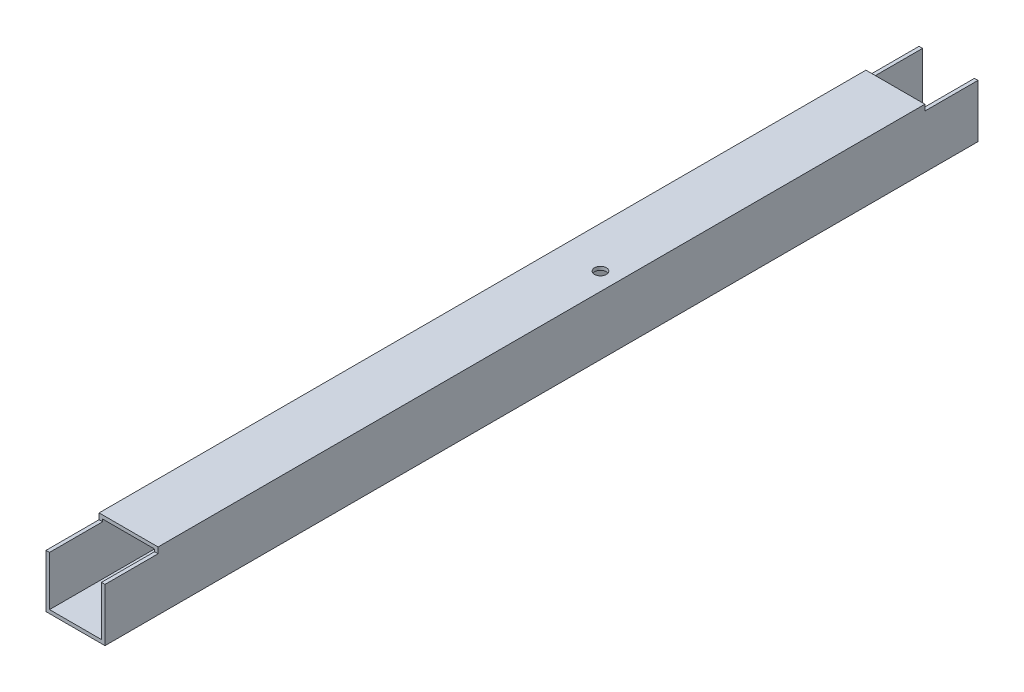
from build123d import *

# Parameters (mm, degrees)
SKETCH_1_W          = 50
SKETCH_1_H          = 50
SKETCH_1_W_2        = 44
SKETCH_1_H_2        = 44
EXTRUDE_1_DEPTH     = 790
SKETCH_2_W          = 50
SKETCH_2_H          = 45
CUT_EXTRUDE_1_DEPTH = 5
SKETCH_3_R          = 5
CUT_EXTRUDE_2_DEPTH = 5
CUT_EXTRUDE_3_DEPTH = 50
CUT_EXTRUDE_4_DEPTH = 50
EXTRUDE_2_DEPTH     = 25
EXTRUDE_3_DEPTH     = 25
CUT_EXTRUDE_5_DEPTH = 25
CUT_EXTRUDE_6_DEPTH = 25
SKETCH_10_R         = 5
CUT_EXTRUDE_7_DEPTH = 94


with BuildPart() as part:
    # 草图1 → 凸台-拉伸1 (new body)
    with BuildSketch(Plane.XY):
        with Locations((25, 25)):
            Rectangle(SKETCH_1_W, SKETCH_1_H)
        with Locations((25, 25)):
            Rectangle(SKETCH_1_W_2, SKETCH_1_H_2, mode=Mode.SUBTRACT)
    extrude(amount=EXTRUDE_1_DEPTH)

    # 草图2 → 切除-拉伸1 (cut)
    with BuildSketch(Plane(origin=(0, 50, 0), x_dir=(1, 0, 0), z_dir=(0, 1, 0))):
        with Locations((25, -22.5)):
            Rectangle(SKETCH_2_W, SKETCH_2_H)
        with Locations((25, -767.5)):
            Rectangle(SKETCH_2_W, SKETCH_2_H)
    extrude(amount=-CUT_EXTRUDE_1_DEPTH, mode=Mode.SUBTRACT)

    # 草图3 → 切除-拉伸2 (cut)
    with BuildSketch(Plane(origin=(0, 50, 0), x_dir=(1, 0, 0), z_dir=(0, 1, 0))):
        with Locations(Location((35, -330, 0), (0, 0, 270))):
            Circle(SKETCH_3_R)
    extrude(amount=-CUT_EXTRUDE_2_DEPTH, mode=Mode.SUBTRACT)

    # 草图4 → 切除-拉伸3 (cut)
    with BuildSketch(Plane.XY.offset(790)):
        Polygon((50, 0), (50, 45), (47, 45), (47, 3), (3, 3), (3, 45), (0, 45), (0, 0), align=None)
    extrude(amount=-CUT_EXTRUDE_3_DEPTH, mode=Mode.SUBTRACT)

    # 草图5 → 切除-拉伸4 (cut)
    with BuildSketch(Plane.XY.offset(745)):
        Polygon((47, 47), (47, 45), (50, 45), (50, 50), (0, 50), (0, 45), (3, 45), (3, 47), align=None)
    extrude(amount=-CUT_EXTRUDE_4_DEPTH, mode=Mode.SUBTRACT)

    # 草图6 → 凸台-拉伸2 (add)
    with BuildSketch(Plane.XY.offset(695)):
        Polygon((3, 47), (47, 47), (47, 45), (50, 45), (50, 50), (0, 50), (0, 45), (3, 45), align=None)
    extrude(amount=EXTRUDE_2_DEPTH)

    # 草图7 → 凸台-拉伸3 (add)
    with BuildSketch(Plane.XY.offset(740)):
        Polygon((0, 0), (50, 0), (50, 45), (47, 45), (47, 3), (3, 3), (3, 45), (0, 45), align=None)
    extrude(amount=EXTRUDE_3_DEPTH)

    # 草图8 → 切除-拉伸5 (cut)
    with BuildSketch(Plane(origin=(0, 0, 0), x_dir=(-1, 0, 0), z_dir=(0, 0, -1))):
        Polygon((0, 0), (0, 45), (-3, 45), (-3, 3), (-47, 3), (-47, 45), (-50, 45), (-50, 0), align=None)
    extrude(amount=-CUT_EXTRUDE_5_DEPTH, mode=Mode.SUBTRACT)

    # 草图9 → 切除-拉伸6 (cut)
    with BuildSketch(Plane(origin=(0, 0, 45), x_dir=(-1, 0, 0), z_dir=(0, 0, -1))):
        Polygon((-47, 45), (-47, 47), (-3, 47), (-3, 45), (0, 45), (0, 50), (-50, 50), (-50, 45), align=None)
    extrude(amount=-CUT_EXTRUDE_6_DEPTH, mode=Mode.SUBTRACT)

    # 草图10 → 切除-拉伸7 (cut)
    with BuildSketch(Plane(origin=(0, 50, 0), x_dir=(1, 0, 0), z_dir=(0, 1, 0))):
        with Locations(Location((35, -330, 0), (0, 0, 270))):
            Circle(SKETCH_10_R)
    extrude(amount=-CUT_EXTRUDE_7_DEPTH, mode=Mode.SUBTRACT)


solid = part.part
